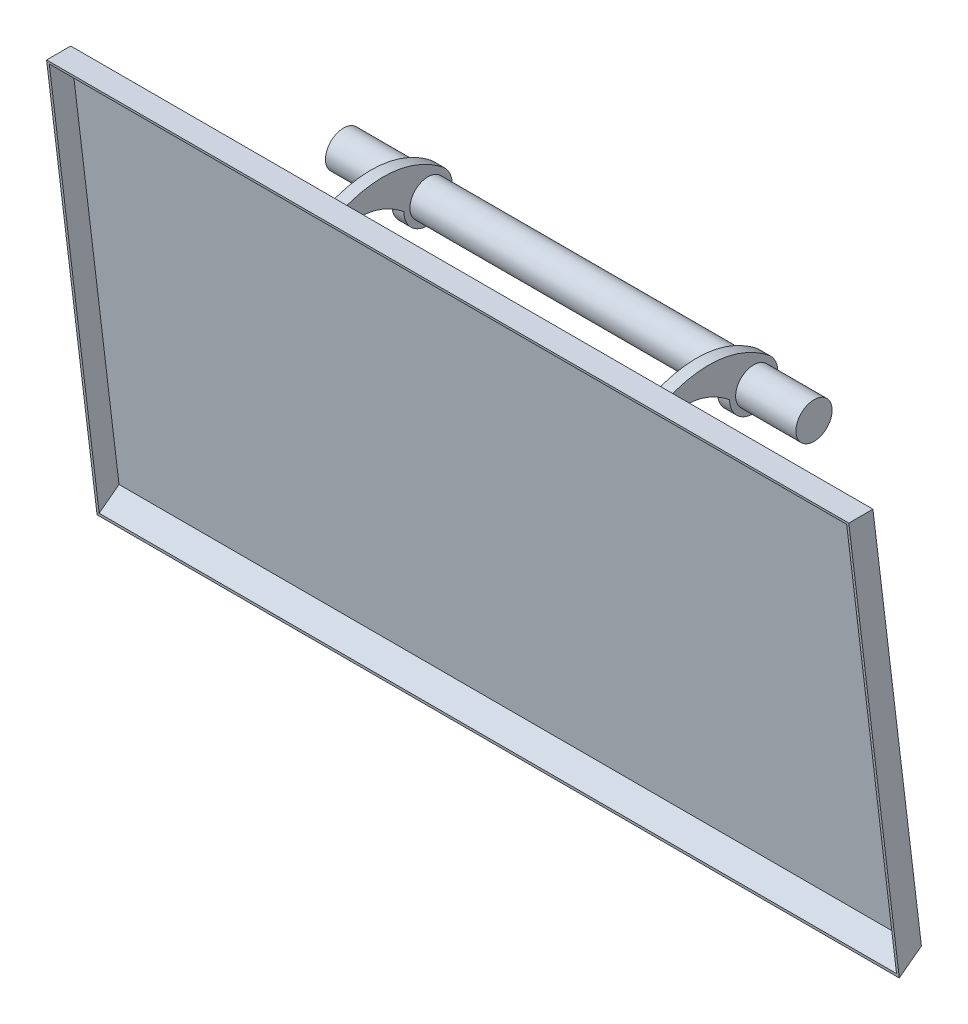
SolidWorks part; units mm, degrees
ref_plane "Front plane" through (0, 0, 0) normal (0, 0, 1) x (1, 0, 0)
ref_plane "Top plane" through (0, 0, 0) normal (0, 1, 0) x (1, 0, 0)
ref_plane "Right plane" through (0, 0, 0) normal (1, 0, 0) x (0, 0, -1)
sketch "Sketch1" plane through (0, 0, 0) normal (1, 0, 0) x (0, 0, -1)
  line L0 (0, 0) -> (-20, 0)
  line L3 (-20, 0) -> (21.8339, -347.4909)
  line L5 (21.8339, -347.4909) -> (40.1779, -333.7355)
  line L9 (40.1779, -333.7355) -> (0, 0)
  dimension "D3" = 350
  dimension "D1" = 20
  dimension "D2" = 120
  dimension "D4" = 96.865
extrude "Boss-Extrude1" add sketch "Sketch1" along normal blind 2
sketch "Sketch2" plane through (0, 0, 0) normal (-1, 0, 0) x (0, 0, 1)
  line L0 (0, 0) -> (20, 0) construction
  line L1 (-40.1779, -333.7355) -> (0, 0) construction
  line L2 (-21.8339, -347.4909) -> (-40.1779, -333.7355) construction
  line L3 (0, 0) -> (20, 0)
  line L4 (-40.1779, -333.7355) -> (0, 0)
  line L5 (-21.8339, -347.4909) -> (-40.1779, -333.7355)
  line L6 (-21.5578, -345.1981) -> (-38.0542, -332.8281)
  line L7 (-38.0542, -332.8281) -> (1.7737, -2)
  line L8 (1.7737, -2) -> (19.7592, -2)
  line L9 (20, 0) -> (-21.8339, -347.4909) construction
  line L10 (20, 0) -> (19.7592, -2)
  line L11 (-21.5578, -345.1981) -> (-21.8339, -347.4909)
  line L12 (-20.634, -345.8908) -> (-38.0542, -332.8281) construction
  line L14 (1.7737, -2) -> (20, -2) construction
  dimension "D1" = 2
extrude "Boss-Extrude2" add sketch "Sketch2" along normal blind 661
sketch "Sketch3" plane through (-661, 0, 0) normal (-1, 0, 0) x (0, 0, 1)
  line L4 (20, 0) -> (0, 0)
  line L5 (-21.8339, -347.4909) -> (20, 0)
  line L6 (-40.1779, -333.7355) -> (-21.8339, -347.4909)
  line L7 (0, 0) -> (-40.1779, -333.7355)
  line L8 (20, 0) -> (0, 0)
  line L9 (-21.8339, -347.4909) -> (20, 0)
  line L10 (-40.1779, -333.7355) -> (-21.8339, -347.4909)
  line L11 (0, 0) -> (-40.1779, -333.7355)
  dimension "D1" = 0
extrude "Boss-Extrude3" add sketch "Sketch3" along normal blind 2
ref_plane "Plane1" through (-195.5, 0, 0) normal (1, 0, 0) x (0, 0, -1)
sketch "Sketch4" plane through (-195.5, 0, 0) normal (1, 0, 0) x (0, 0, -1)
  line L0 (7.2744, -60.4244) -> (3.6074, -29.9648)
  line L1 (40.1779, -333.7355) -> (0, 0) construction
  line L2 (14.3804, -52.5184) -> (12.8261, -39.6083)
  line L3 (15.217, -59.4682) -> (11.5501, -29.0086) construction
  line L4 (7.2744, -60.4244) -> (8.2672, -60.3049)
  circle A0 centre (88.6694, -49.4664) radius 15
  circle A1 centre (88.6694, -49.4664) radius 20
  arc A2 (14.3804, -52.5184) -> (8.2672, -60.3049) centre (7.4305, -53.3551) cw
  spline S0 degree 2 poles (12.8261, -39.6083) (40.7944, -27.323) (68.6694, -49.4664) knots 0 0 0 1 1 1
  spline S1 degree 3 poles (3.6074, -29.9648) (33.4234, -12.4126) (69.251, -8.887) (100.9912, -33.7128) knots 0 0 0 0 1 1 1 1
  dimension "D1" = 30
  dimension "D2" = 40
  dimension "D4" = 7
  dimension "D3" = 8
extrude "Boss-Extrude4" add sketch "Sketch4" along normal blind 10
pattern_linear "LPattern1" count 2 spacing 270 along (-1, 0, 0) of "Boss-Extrude4"
sketch "Sketch5" plane through (-185.5, 0, 0) normal (1, 0, 0) x (0, 0, -1)
  circle A0 centre (88.6694, -49.4664) radius 15 construction
  circle A1 centre (88.6694, -49.4664) radius 15
extrude "Boss-Extrude5" add sketch "Sketch5" against normal blind 340 separate body
sketch "Sketch6" plane through (-185.5, 0, 0) normal (1, 0, 0) x (0, 0, -1)
  circle A1 centre (88.6694, -49.4664) radius 15
  circle A2 centre (88.6694, -49.4664) radius 15
  dimension "D1" = 0
extrude "Boss-Extrude6" add sketch "Sketch6" along normal blind 50
